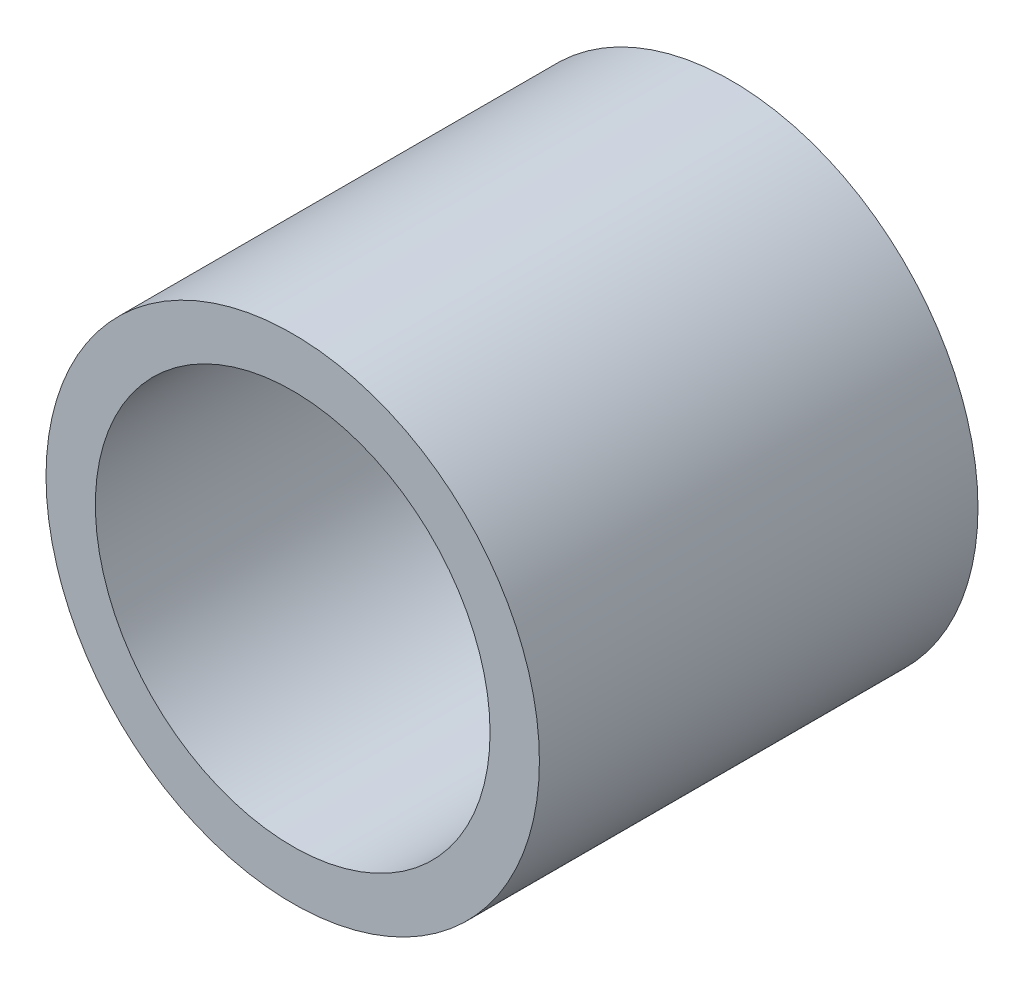
from build123d import *

# Parameters (mm, degrees)
SKETCH_1_R      = 45
SKETCH_1_R_2    = 36
EXTRUDE_1_DEPTH = 40


with BuildPart() as part:
    # 草图1 → 凸台-拉伸1 (new, symmetric)
    with BuildSketch(Plane.XY):
        Circle(SKETCH_1_R)
        Circle(SKETCH_1_R_2, mode=Mode.SUBTRACT)
    extrude(amount=EXTRUDE_1_DEPTH, both=True)


solid = part.part
